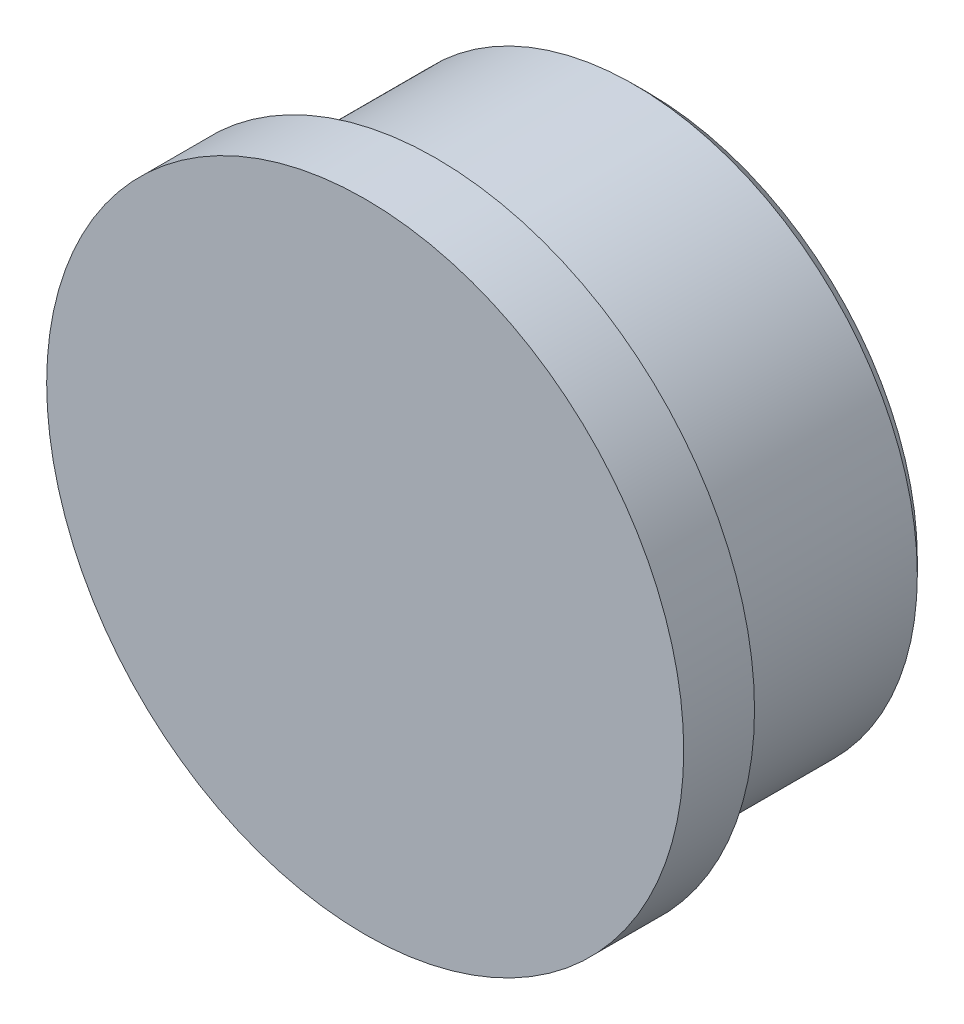
SolidWorks part; units mm, degrees
material "Q345 "
ref_plane "前视基准面" through (0, 0, 0) normal (0, 0, 1) x (1, 0, 0)
ref_plane "上视基准面" through (0, 0, 0) normal (0, 1, 0) x (1, 0, 0)
ref_plane "右视基准面" through (0, 0, 0) normal (1, 0, 0) x (0, 0, -1)
sketch "草图1" plane through (0, 0, 0) normal (0, 0, 1) x (1, 0, 0)
  circle A0 centre (0, 0) radius 40
  dimension "D1" = 80
extrude "凸台-拉伸1" add sketch "草图1" along normal blind 30
sketch "草图2" plane through (0, 0, 30) normal (0, 0, 1) x (1, 0, 0)
  circle A0 centre (0, 0) radius 45
  dimension "D1" = 90
extrude "凸台-拉伸2" add sketch "草图2" along normal blind 10
chamfer "倒角1" distance 2 angle 45 1 edges at (40, 0, 0)
